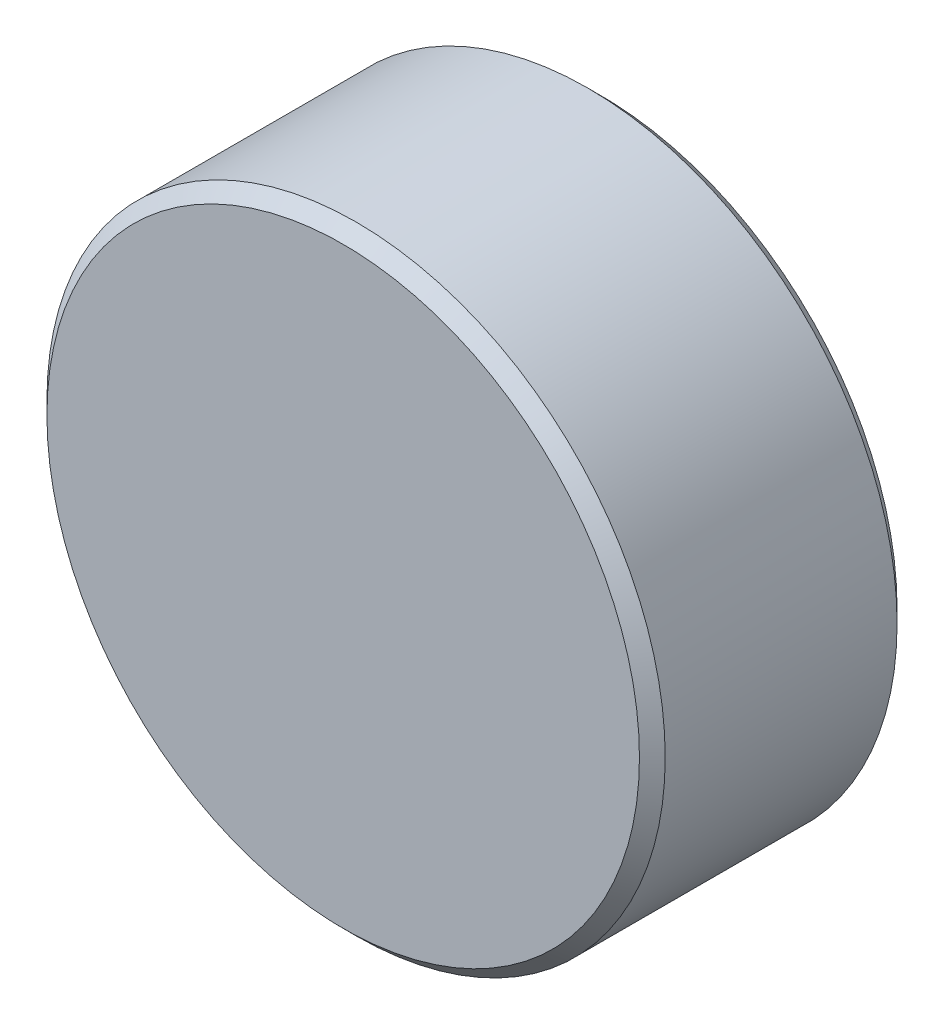
SolidWorks part; units mm, degrees
ref_plane "前视基准面" through (0, 0, 0) normal (0, 0, 1) x (1, 0, 0)
ref_plane "上视基准面" through (0, 0, 0) normal (0, 1, 0) x (1, 0, 0)
ref_plane "右视基准面" through (0, 0, 0) normal (1, 0, 0) x (0, 0, -1)
sketch "草图1" plane through (0, 0, 0) normal (0, 0, 1) x (1, 0, 0)
  circle A0 centre (0, 0) radius 12
  dimension "D1" = 24
extrude "凸台-拉伸1" add sketch "草图1" along normal blind 10
cosmetic thread "装饰螺纹线2" parameters "D2"=21.835
chamfer "倒角1" distance 0.5 angle 45 2 edges at (12, 0, 0) (12, 0, 10)
sketch "草图2" plane through (0, 0, 0) normal (0, 0, -1) x (-1, 0, 0)
  line L0 (0, 0) -> (-8.9688, 0) construction
  line L1 (0, -3.4641) -> (3, -1.7321)
  line L2 (3, -1.7321) -> (3, 1.7321)
  line L3 (3, 1.7321) -> (0, 3.4641)
  line L4 (0, 3.4641) -> (-3, 1.7321)
  line L5 (-3, 1.7321) -> (-3, -1.7321)
  line L6 (-3, -1.7321) -> (0, -3.4641)
  circle A0 centre (0, 0) radius 3 construction
  dimension "D1" = 6
extrude "切除-拉伸1" cut sketch "草图2" against normal blind 8
